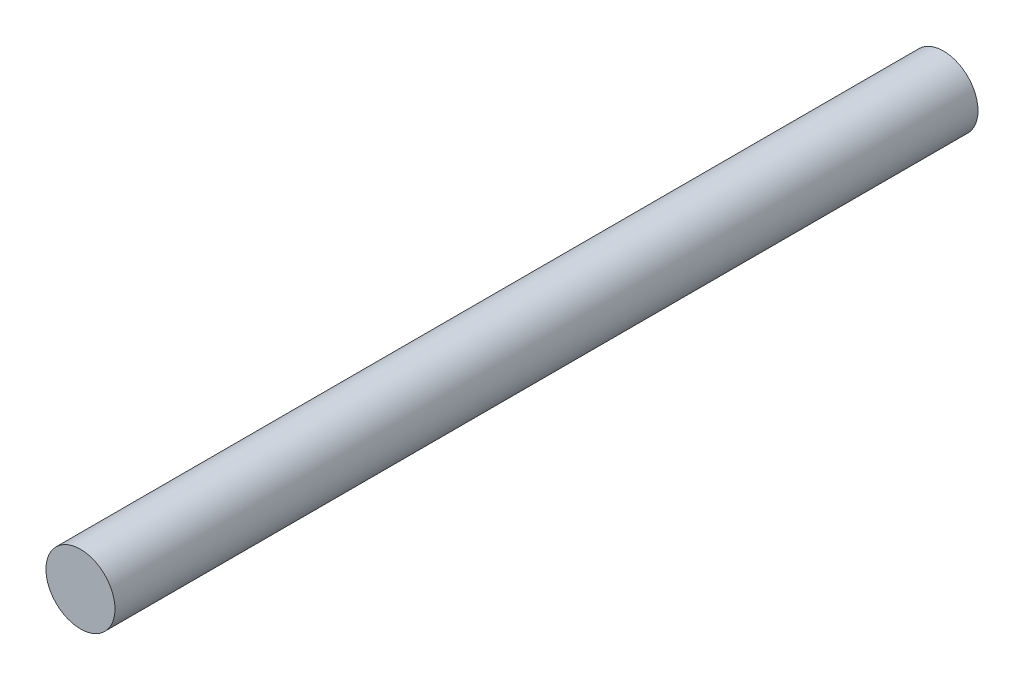
from build123d import *

# Parameters (mm, degrees)
SKETCH_1_R      = 6
EXTRUDE_1_DEPTH = 75


with BuildPart() as part:
    # 草图1 → 凸台-拉伸1 (new, symmetric)
    with BuildSketch(Plane.XY):
        Circle(SKETCH_1_R)
    extrude(amount=EXTRUDE_1_DEPTH, both=True)


solid = part.part
